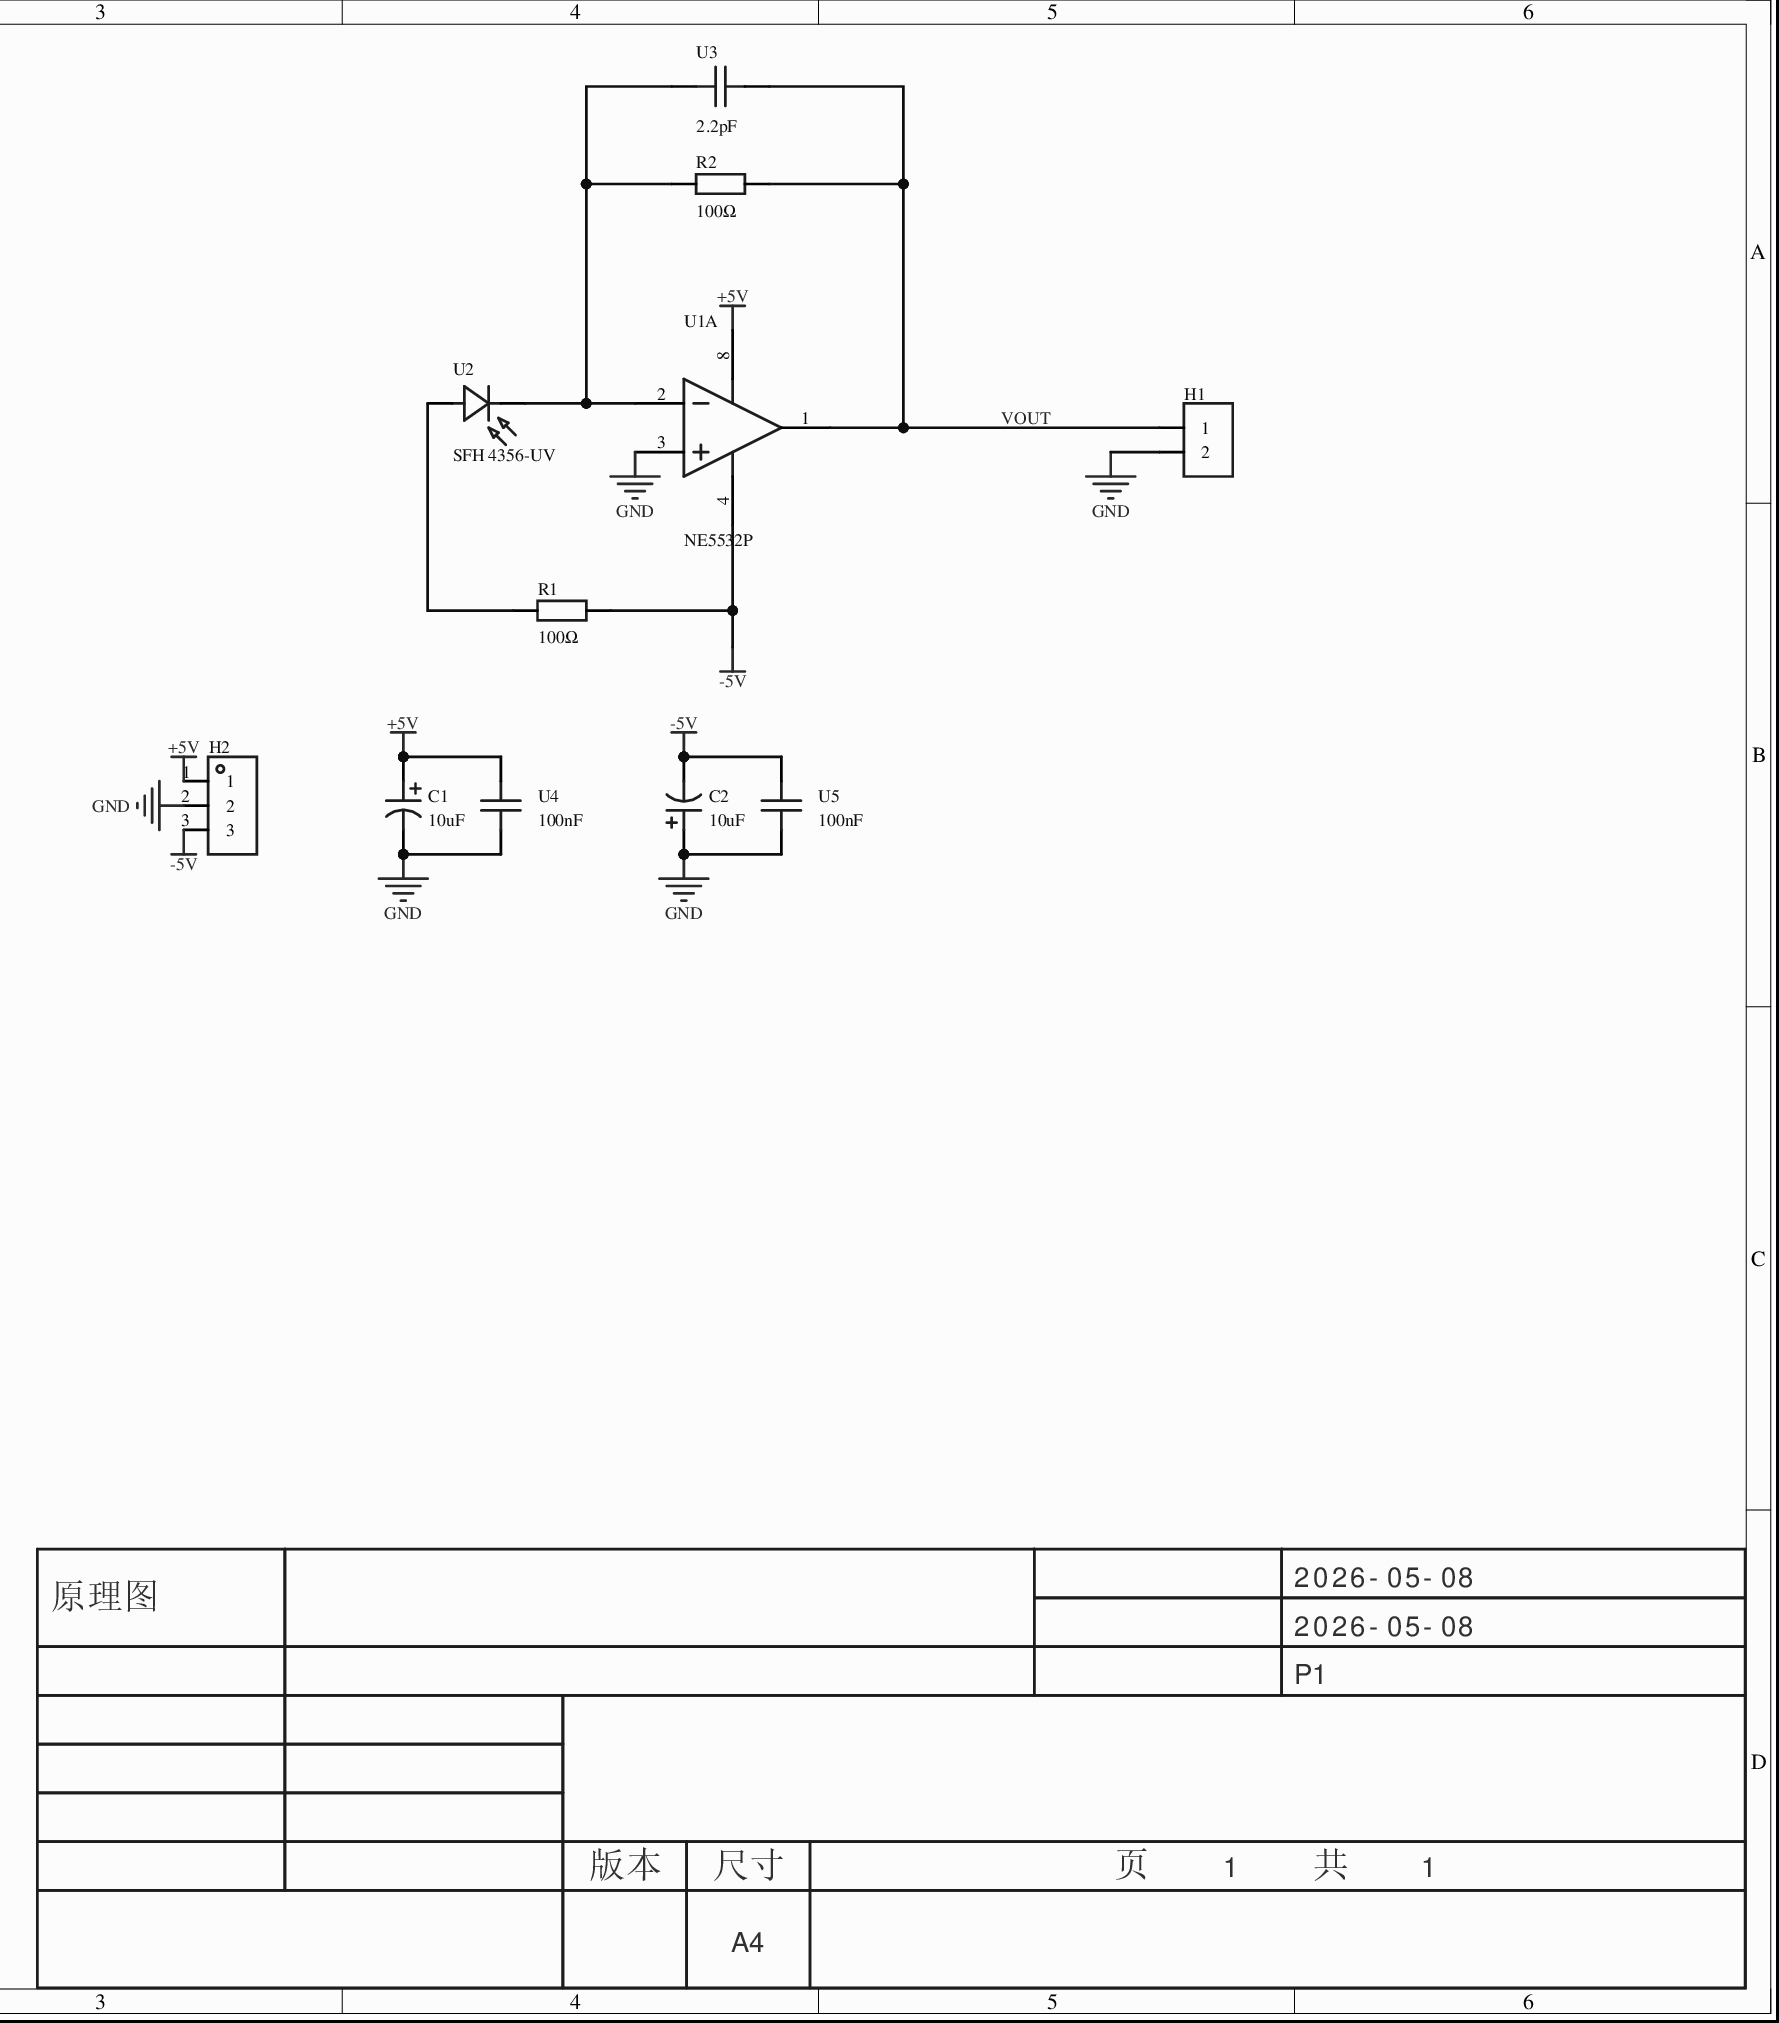
[diagram p0: MISC51879-3.schdoc]
# Altium project MISC51879-2.PrjPcb
1 sheet, 11 parts. Net scope: global (net labels, ports and power ports of the same name join across sheets).
Board file: MISC51879.pcbdoc

## Sheet MISC51879-3.schdoc
size 297 x 209 mm; Version: V1.0; @Project Name: MISC51879; @Update Date: 2026-05-08; @Create Date: 2026-05-08; @Board Name: MISC51879; @Create Time: 10:20:54; @Page Count: 1; @Page No: 1; @Schematic Name: MISC51879; @Update Time: 10:20:54; Size: A4

### Parts
C1  10uF  [CAP-TH_BD5.0-P2.00-D0.8-FD-10UF50VC110GL]
C2  10uF  [CAP-TH_BD5.0-P2.00-D0.8-FD-10UF50VC110GL]
H1  (no value)  [HDR-TH_2P-P2.54-V-F]
H2  (no value)  [HDR-TH_3P-P2.54-V-F]
R1  100Ω  [Res_1/8W]
R2  100Ω  [Res_1/8W]
U1  NE5532P  [DIP-8_L9.4-W6.4-P2.54-LS9.1-BL]  (part A of 2)
U2  SFH 4356-UV  [LED-TH_BD3.8-P2.54-FD]
U3  2.2pF  [CAP-TH_L5.0-W2.5-P5.00-D1.0]
U4  100nF  [CAP-TH_L5.0-W2.5-P5.00-D1.0]
U5  100nF  [CAP-TH_L5.0-W2.5-P5.00-D1.0]

### Nets
+5V: C1.1 H2.1 U1.8(VCC+) U4.1
-5V: C2.2 H2.3 R1.2 U1.4(VCC-) U5.1
GND: C1.2 C2.1 H1.2 H2.2 U1.3(IN1+) U4.2 U5.2
VOUT: H1.1 R2.2 U1.1(OUT1) U3.1
NetR1_1: R1.1 U2.1(A)
NetR2_1: R2.1 U1.2(IN1-) U2.2(C) U3.2

### Notes on the sheet
- 2026-05-08
- 原理图
- P1
- 版本
- 尺寸
- A4
- 页    1    共    1

### Library data of the parts
C1 C2 = 10UF50VC110GL: 容值:10uF;精度:±20%;额定电压:50V;纹波电流:120mA@100KHz;等效串联电阻(ESR):1.6Ω;; Manufacturer: Econd(米朗电子); AddInBom: yes; Tolerance: ±20%; Voltage Rating: 50V; Equivalent Series Resistance(ESR): 1.6Ω; Pin Spacing: 2mm; Lifetime: 5000hrs@105℃; Symbol: 10UF50VC110GL; Device: 10UF50VC110GL; LCSC Part Name: 10uF ±20% 50V; SupplierPart: C46867109; ManufacturerPart: 10UF50VC110GL; Supplier Footprint: 插件,D5xL11mm; JLCPCB Part Class: Extended Part; Datasheet: https://item.szlcsc.com/datasheet/10UF50VC110GL/49031974.html; Supplier: LCSC; ConvertToPcb: yes; FootprintName: CAP-TH_BD5.0-P2.00-D0.8-FD-10UF50VC110GL; Value: 10uF; Ripple Current: 120mA@100KHz; Diameter: 5mm; Height - Seated (Max): 11mm; Operating Temperature: -40℃~+105℃
H1 = HDR-F_2.54_1x2P: Symbol: Header-Female-2.54_1x2; ConvertToPcb: yes; ModelId: a9450ef445564560a104363b9aacde4e0819f05c4eef4c71ace90d822a990e87; ModelName: HDR-TH_2P-P2.54-F-LI-1X2P; ModelTransform: 215.7476,98.425,0,0,0,0,0,0,-129.921; Device: HDR-F_2.54_1x2P; AddInBom: yes; SupplierPart: C49661; Supplier Footprint: 插件; FootprintName: HDR-TH_2P-P2.54-V-F
H2 = HDR-F_2.54_1x3P: Symbol: PM254V-11-03-H85; ConvertToPcb: yes; ModelId: f3b3cc5aae9641bf9e56fc160cef875b0819f05c4eef4c71ace90d822a990e87; ModelName: HDR2.54-F-LI-1X3P; ModelTransform: 299.9994,100,0,0,0,0,0,0,-118.11; Device: HDR-F_2.54_1x3P; AddInBom: yes; SupplierPart: C541850; Supplier Footprint: 插件; FootprintName: HDR-TH_3P-P2.54-V-F
R1 R2 = Res_AXIAL-1/8W: Symbol: 电阻; ConvertToPcb: yes; ModelId: b2b5ae7ae4c642178fe0039925c86a3f0819f05c4eef4c71ace90d822a990e87; ModelName: RES-TH_BD1.8-L3.2-P7.20-D0.4; ModelTransform: 282.86,66.88,253.09,0,0,0,0,0,-191; Device: Res_AXIAL-1/8W; Value: 100Ω; AddInBom: yes; Supplier Footprint: 轴向引线; FootprintName: Res_1/8W
U1 = NE5532P: 放大器数:2;轨到轨:-;增益带宽积(GBW):10MHz;输入失调电压(Vos):4mV;压摆率(SR):9V/us;输入偏置电流(Ib):1uA;; Manufacturer: TI(德州仪器); Relevance: []; AddInBom: yes; ModelId: 5746b540d01a4d1b9eb6b4f989297bc70819f05c4eef4c71ace90d822a990e87; ModelName: DIP-8_L9.8-W6.6-H3.5-LS7.62-P2.54; ModelTransform: 385.826,311.8104,0,0,0,0,0,-0.0005,-118.11; Number of Channels: 2; Maximum Power Supply Range (Vdd-Vss): 30V; Gain Bandwidth Product: 10MHz; Vos - Input Offset Voltage: 4mV; Input Offset Voltage Drift(Vos TC): 5uV/℃; Slew Rate: 9V/us; Ib - Input Bias Current: 1uA; Input Offset Current(Ios): 150nA; Input Voltage Noise Density: 5nV/√Hz@1kHz; Common Mode Rejection Ratio(CMRR): 100dB; Quiescent Current: 16mA; Output Current: 38mA; Dual Supply: -15V~15V; Symbol: NE5532P; Device: NE5532P; LCSC Part Name: 低噪声双运放; SupplierPart: C5326; ManufacturerPart: NE5532P; Supplier Footprint: PDIP-8; JLCPCB Part Class: Extended Part; Datasheet: https://www.ti.com/cn/lit/gpn/ne5532; Supplier: LCSC; ConvertToPcb: yes; FootprintName: DIP-8_L9.4-W6.4-P2.54-LS9.1-BL; Rail to Rail: -; Input offset current drift(Ios TC): -; Operating Temperature: 0℃~+70℃; Single supply: -
U2 = SFH 4356-UV: 正向电压:1.7V;波长:860nm;辐射强度:40mW/sr@100mA;视角:40°;; Manufacturer: OSRAM(欧司朗); AddInBom: yes; ModelId: 7a5158147ccf41a18926a05cf5a7749d0819f05c4eef4c71ace90d822a990e87; ModelTransform: 139.516,157.15173,0,0,0,0,-9.054,-1.181,-137.795; Vf - Forward Voltage: 1.7V; Wavelength: 860nm; View Angle: 40°; Symbol: SFH 4356-UV; Device: SFH 4356-UV; LCSC Part Name: 光电二极管; SupplierPart: C2900361; ManufacturerPart: SFH 4356-UV; Supplier Footprint: 插件; JLCPCB Part Class: Extended Part; Supplier: LCSC; ConvertToPcb: yes; FootprintName: LED-TH_BD3.8-P2.54-FD; ModelName: LED-TH_BD3.8-P2.54-FD; Radiant Intensity: 40mW/sr@100mA; Operating Temperature: -40℃~+100℃
U3-U5 = 100nF: Symbol: 100NF_C9900015256; AddInBom: yes; ModelId: 08e3d7481fc7486bb1b263873f51e1e10819f05c4eef4c71ace90d822a990e87; ModelName: CAP-TH_BD5.0-W2.5-P5.08; ModelTransform: 224.652,98.425,0,0,0,0,-0.005,0,-137.795; Device: 100nF; LCSC Part Name: 100nF; SupplierPart: C9900015256; Supplier Footprint: CAP-TH_L5.0-W2.5-P5.00-D1.0; JLCPCB Part Class: Extended Part; Supplier: LCSC; ConvertToPcb: yes; FootprintName: CAP-TH_L5.0-W2.5-P5.00-D1.0
  U3: Manufacturer Part: 2.2pF
  U4 U5: ManufacturerPart: 100nF